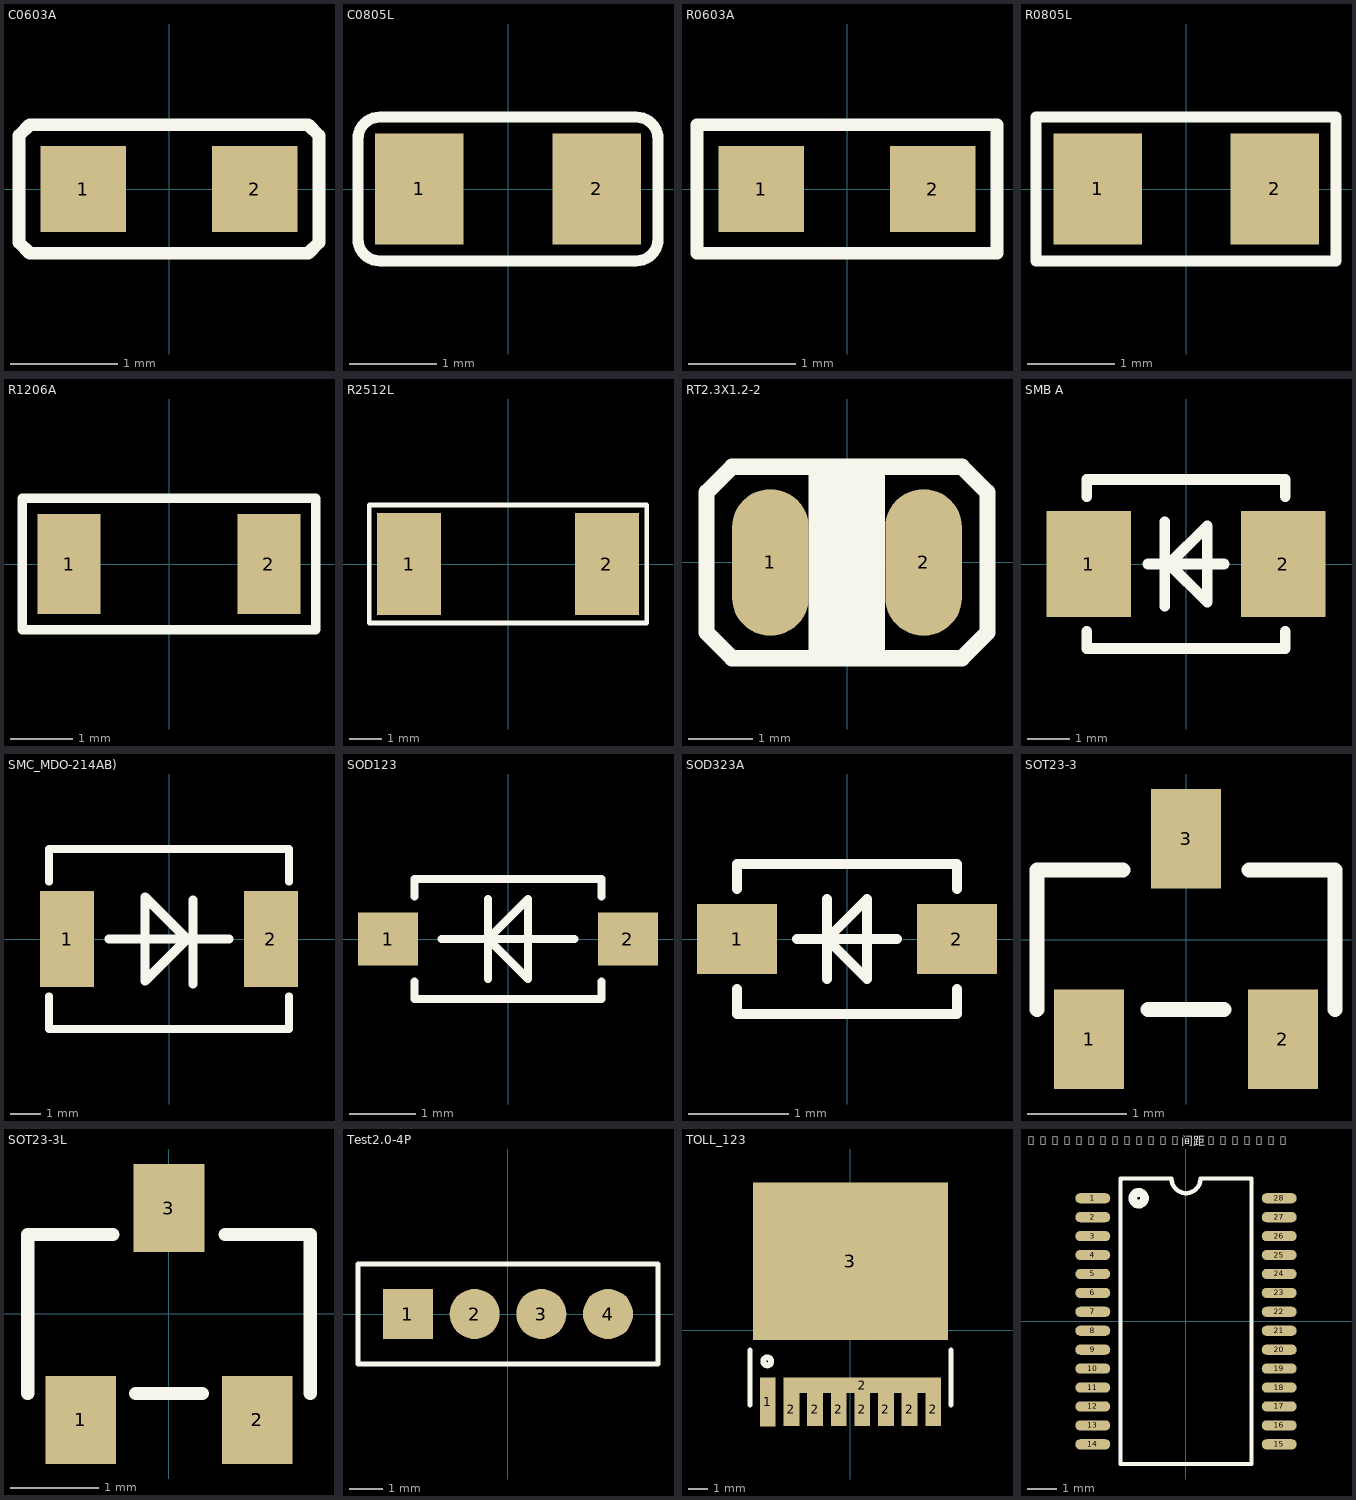
[diagram p0: the footprints below, top view; thin cyan lines are the x and y axes]
# Altium footprint library MISC82749.PcbLib: 16 footprints
Each footprint in its own frame and in the unit in brackets; x right, y up, seen from the top. Pads: shape width x height; smd on the part's side, far side on the other; paste and mask are expansions set on the pad; w line width, h text height; cw(c..) or ccw(c..) is an arc to the next point about the centre after c.

## C0603A [mm] "SMD capacitor"
pads (2):
  rect 0.8x0.8 smd mask+0.08: 1(-0.8,0) 2(0.8,0)
Top Overlay:
  lines w0.12: 0.551,-0.6 1.2,-0.6 ; -1.4,-0.5 -1.4,0.5 -1.3,0.6 1.3,0.6 1.4,0.5 1.4,-0.5 1.3,-0.6 -1.3,-0.6 -1.4,-0.5

## C0805L [mil] "SMD capacitor"
pads (2):
  rect 40x50 smd paste+0 mask+1.97: 1(-40,0) 2(40,0)
Top Overlay:
  lines w5: -67.72,-22.64 ccw(c-57.87,-22.64) -57.87,-32.48 57.87,-32.48 ccw(c57.87,-22.64) 67.72,-22.64 67.72,22.64 ccw(c57.87,22.64) 57.87,32.48 -57.87,32.48 ccw(c-57.87,22.64) -67.72,22.64 -67.72,-22.64

## R0603A [mm] "SMD resistor"
height 0.5
pads (2):
  rect 0.8x0.8 smd mask+0.08: 1(-0.8,0) 2(0.8,0)
Top Overlay:
  lines w0.12: -1.4,-0.6 -1.4,0.6 1.4,0.6 1.4,-0.6 -1.4,-0.6

## R0805L [mil] "SMD resistor"
pads (2):
  rect 40x50 smd paste+0 mask+1.97: 1(-40,0) 2(40,0)
Top Overlay:
  lines w5: -67.91,-32.48 -67.91,32.48 ; -67.72,-32.48 67.72,-32.48 67.72,32.48 -67.72,32.48

## R1206A [mm] "SMD resistor"
pads (2):
  rect 1x1.6 smd: 1(-1.6,0) 2(1.6,0)
Top Overlay:
  lines w0.15: -2.35,-1.05 -2.35,1.05 2.35,1.05 2.35,-1.05 -2.35,-1.05

## R2512L [mm] "SMD resistor"
pads (2):
  rect 2x3.2 smd: 1(-3.1,0) 2(3.1,0)
Top Overlay:
  lines w0.15: -4.35,-1.85 -4.35,1.85 4.35,1.85 4.35,-1.85 -4.35,-1.85

## RT2.3X1.2-2 [mm] "wire-lead NTC"
pads (2):
  oval 1.2x2.3 smd: 1(-1.2,0) 2(1.2,0)
Top Overlay:
  rectangle: -0.601,-1.55 0.599,1.5
  lines w0.254: -2.2,-1.075 -2.2,1.075 ; -2.2,1.1 -1.8,1.5 ; 2.2,-1.075 2.2,1.075 ; 2.2,1.1 1.8,1.5 -1.8,1.5 ; -2.2,-1.1 -2.2,-1.1 ; -2.2,-1.1 -1.8,-1.5 ; -1.8,-1.5 1.8,-1.5 2.2,-1.1 ; -1.8,-1.5 -1.8,-1.5 ; -1.8,1.5 -1.8,1.5 ; 2.2,-1.1 2.2,-1.1

## SMB A [mm] "SMD diode"
pads (2):
  rect 2x2.5 smd: 1(-2.3,0) 2(2.3,0)
Top Overlay:
  lines w0.254: -2.35,-1.6 -2.35,-2 2.35,-2 2.35,-1.6 ; -2.35,1.6 -2.35,2 2.35,2 2.35,1.6 ; -0.9,0 0.9,0 ; -0.5,-1 -0.5,1 ; -0.4,0 0.5,-0.9 0.5,0.9 -0.4,0

## SMC_MDO-214AB) [mm] "SMD diode"
pads (2):
  rect 1.8x3.2 smd: 1(-3.4,0) 2(3.4,0)
Top Overlay:
  lines w0.254: -4,-1.905 -4,-3 4,-3 4,-1.905 ; -4,1.905 -4,3 4,3 4,1.905
  lines w0.3: -2,0 2,0 ; 0.8,-1.5 0.8,1.3 ; -0.8,-1.4 0.6,0 -0.8,1.4 -0.8,-1.4

## SOD123 [mm] "SMD diode"
pads (2):
  rect 0.9x0.8 smd: 1(-1.8,0) 2(1.8,0)
Top Overlay:
  lines w0.12: -1.4,-0.635 -1.4,-0.9 1.4,-0.9 1.4,-0.635 ; -1.4,0.635 -1.4,0.9 1.4,0.9 1.4,0.635 ; -1,0 1,0 ; -0.3,-0.602 -0.3,0.6 ; -0.3,0 0.3,-0.6 0.3,0.6 -0.3,0

## SOD323A [mm] "SMD diode"
pads (2):
  rect 0.8x0.7 smd: 1(-1.1,0) 2(1.1,0)
Top Overlay:
  lines w0.1: -1.1,-0.5 -1.1,-0.75 1.1,-0.75 1.1,-0.5 ; -1.1,0.5 -1.1,0.75 1.1,0.75 1.1,0.5 ; -0.5,0 0.5,0 ; -0.2,-0.4 -0.2,0.4 ; -0.2,0 0.2,-0.4 0.2,0.4 -0.2,0

## SOT23-3 [mm] "SMD IC/MOS*"
pads (3):
  rect 0.7x1 smd: 1(-0.975,-1) 2(0.975,-1) 3(0,1.016)
Top Overlay:
  lines w0.15: -1.5,-0.7 -1.5,0.7 -0.635,0.7 ; -0.381,-0.7 0.381,-0.7 ; 0.635,0.7 1.5,0.7 1.5,-0.7

## SOT23-3L [mm] "SMD MOSFET"
pads (3):
  rect 0.8x1 smd: 1(-1,-1.2) 2(1,-1.2) 3(0,1.2)
Top Overlay:
  lines w0.15: -1.6,-0.9 -1.6,0.9 -0.635,0.9 ; -0.381,-0.9 0.381,-0.9 ; 0.635,0.9 1.6,0.9 1.6,-0.9

## Test2.0-4P [mm] "test socket 2.0mm"
pads (4):
  rect 1.5x1.5 smd: 1(-3,0)
  round 1.5 smd: 2(-1,0) 3(1,0) 4(3,0)
Top Overlay:
  lines w0.15: -4.5,-1.5 4.5,-1.5 4.5,1.5 -4.5,1.5 -4.5,-1.5

## TOLL_123 [mm] "SMD MOSFET"
height 3.35
pads (10):
  rect 0.8x2.5 smd: 1(-4.2,-3.638)
  rect 0.8x1.7 smd: 2(-3,-4) 2(-1.8,-4) 2(-0.6,-4) 2(0.6,-4) 2(1.8,-4) 2(3,-4) 2(4.2,-4)
  rect 8x0.8 smd: 2(0.6,-2.788)
  rect 9.9x8 smd: 3(0,3.5)
Top Overlay:
  circle w0.3: c-4.225,-1.575 r0.2
  lines w0.254: -5.1,-3.8 -5.1,-1 ; 5.1,-3.8 5.1,-1
Top Paste:
  region: -3.4,-3.03 -3.4,-2.39 4.6,-2.39 4.6,-3.08
  region: -4.95,7.5 4.95,7.5 4.95,-0.5 -4.95,-0.5
  region: -4.6,-4.85 -4.6,-3.15 -3.8,-3.15 -3.8,-4.85
  region: 3.8,-4.85 3.8,-3.25 4.6,-3.25 4.6,-4.85
  region: 2.6,-4.85 2.6,-3.25 3.4,-3.25 3.4,-4.85
  region: 1.4,-4.85 1.4,-3.25 2.2,-3.25 2.2,-4.85
  region: 0.2,-4.85 0.2,-3.25 1,-3.25 1,-4.85
  region: -1,-4.85 -1,-3.25 -0.2,-3.25 -0.2,-4.85
  region: -2.2,-4.85 -2.2,-3.25 -1.4,-3.25 -1.4,-4.85
  region: -3.4,-4.85 -3.4,-3.25 -2.6,-3.25 -2.6,-4.85

## TSSOP-28L(PIN间距0.65mm) [mm] "SMD IC"
pads (28):
  oval 1.2x0.35 smd: 1(-3.2,4.225) 2(-3.2,3.575) 3(-3.2,2.925) 4(-3.2,2.275) 5(-3.2,1.625) 6(-3.2,0.975) 7(-3.2,0.325) 8(-3.2,-0.325) 9(-3.2,-0.975) 10(-3.2,-1.625) 11(-3.2,-2.275) 12(-3.2,-2.925) 13(-3.2,-3.575) 14(-3.2,-4.225) 15(3.2,-4.225) 16(3.2,-3.575) 17(3.2,-2.925) 18(3.2,-2.275) 19(3.2,-1.625) 20(3.2,-0.975) 21(3.2,-0.325) 22(3.2,0.325) 23(3.2,0.975) 24(3.2,1.625) 25(3.2,2.275) 26(3.2,2.925) 27(3.2,3.575) 28(3.2,4.225)
Top Overlay:
  circle w0.3: c-1.625,4.225 r0.2
  lines w0.15: -2.237,4.854 -2.191,4.9 ; -2.25,-4.9 2.25,-4.9 2.25,4.9 0.5,4.9 cw(c0,4.9) -0.5,4.9 -2.25,4.9 -2.25,-4.9